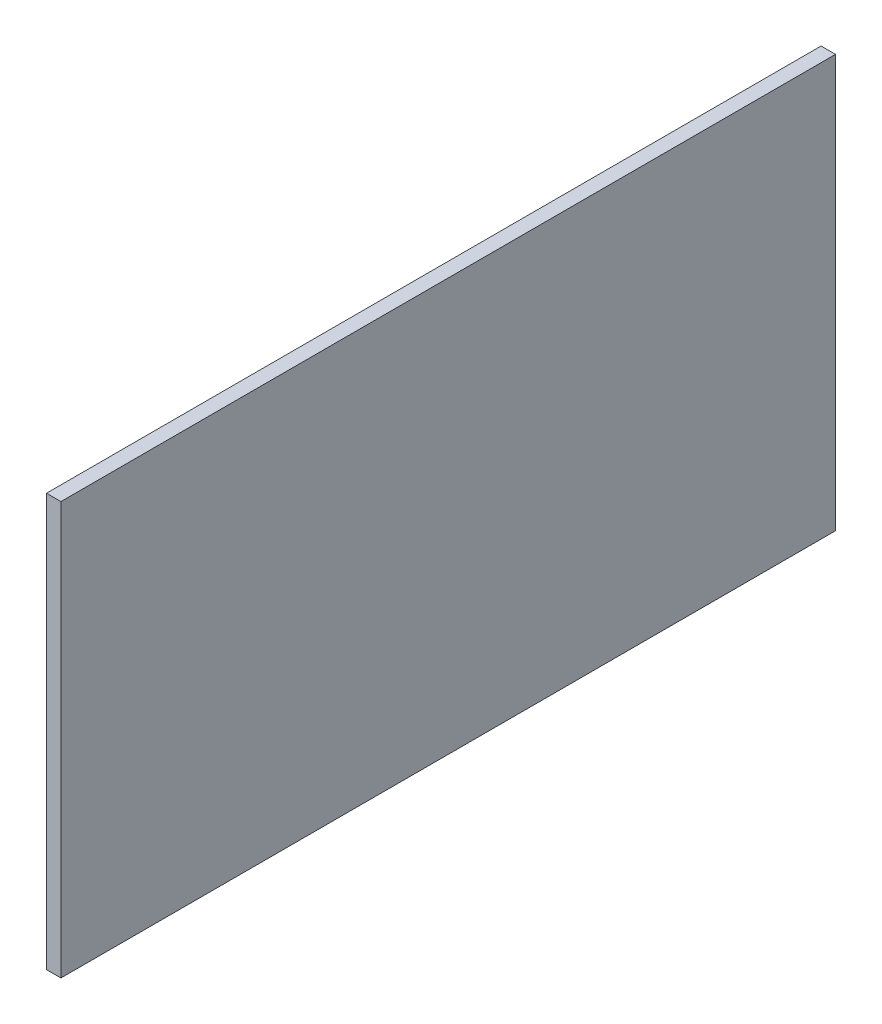
from build123d import *

# Parameters (mm, degrees)
SKETCH1_W           = 563.2
SKETCH1_H           = 300
BOSS_EXTRUDE1_DEPTH = 10.5


with BuildPart() as part:
    # Sketch1 → Boss-Extrude1 (new body)
    with BuildSketch(Plane(origin=(0, 0, 0), x_dir=(0, 0, -1), z_dir=(1, 0, 0))):
        with Locations((281.6, 150)):
            Rectangle(SKETCH1_W, SKETCH1_H)
    extrude(amount=BOSS_EXTRUDE1_DEPTH)


solid = part.part
